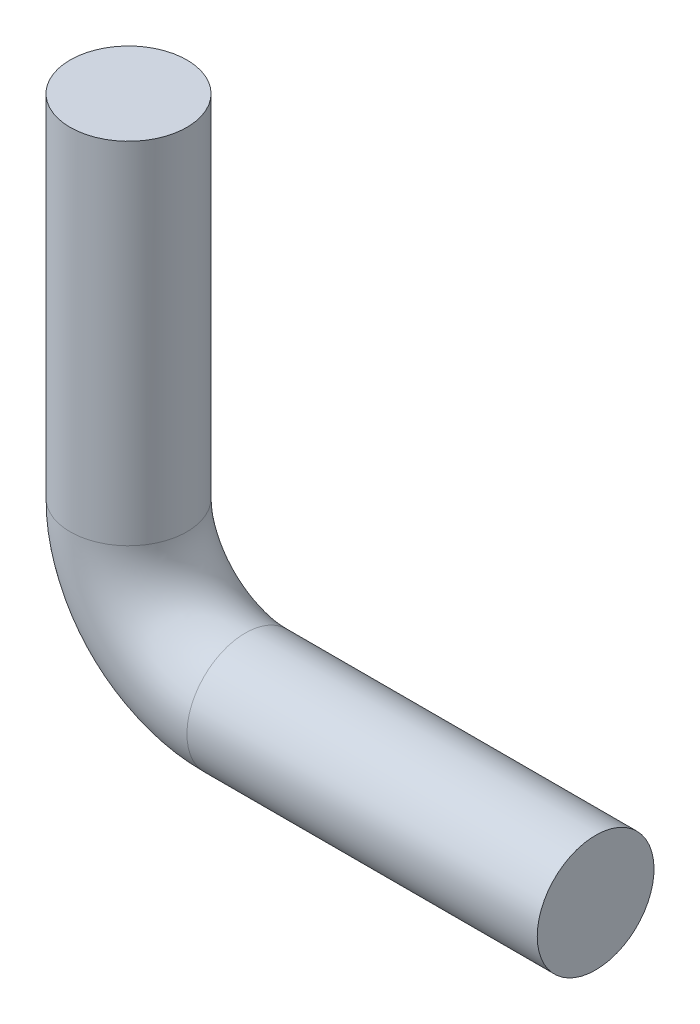
SolidWorks part; units mm, degrees
ref_plane "Front Plane" through (0, 0, 0) normal (0, 0, 1) x (1, 0, 0)
ref_plane "Top Plane" through (0, 0, 0) normal (0, 1, 0) x (1, 0, 0)
ref_plane "Right Plane" through (0, 0, 0) normal (1, 0, 0) x (0, 0, -1)
sketch "Sketch1" plane through (0, 0, 0) normal (0, 0, 1) x (1, 0, 0)
  line L6 (-42.3943, -24.2385) -> (-4.2943, -24.2385)
  line L7 (-55.0943, 26.5615) -> (-55.0943, -11.5385)
  arc A1 (-55.0943, -11.5385) -> (-42.3943, -24.2385) centre (-42.3943, -11.5385) ccw
sketch3d "3DSketch1"
sketch "Sketch2" plane through (-4.2943, 0, 0) normal (-1, 0, 0) x (0, 0, 1)
  line L0 (0, -24.2385) -> (0, -11.5385) construction
  circle A0 centre (0, -24.2385) radius 6.35
  dimension "D1" = 12.7
sweep "Sweep8" add profiles "Sketch2" path "Sketch1"
